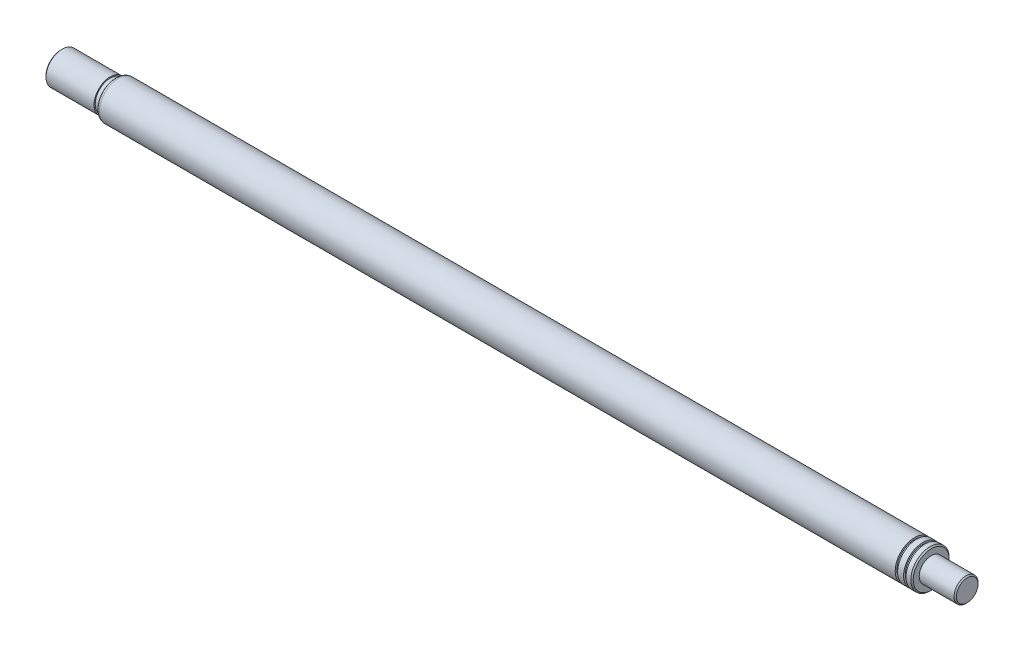
from build123d import *


with BuildPart() as part:
    # 草图1 → 旋转1 (revolve)
    with BuildSketch(Plane.XY, mode=Mode.PRIVATE) as revolve_1_sk:
        with BuildLine():
            Line((0, 0), (0, 12.5))
            Line((0, 12.5), (1, 13.5))
            Line((1, 13.5), (41, 13.5))
            Line((41, 13.5), (41, 12.5))
            Line((41, 12.5), (45, 12.5))
            Line((45, 12.5), (45, 13))
            ThreePointArc((45, 13), (45.878679656, 15.121320344), (48, 16))
            Line((48, 16), (711, 16))
            Line((711, 16), (711, 14.5))
            Line((711, 14.5), (713, 14.5))
            Line((713, 14.5), (713, 16))
            Line((713, 16), (718, 16))
            Line((718, 16), (718, 14.5))
            Line((718, 14.5), (720, 14.5))
            Line((720, 14.5), (720, 16))
            Line((720, 16), (724, 16))
            Line((724, 16), (725, 15))
            Line((725, 15), (725, 10))
            Line((725, 10), (754, 10))
            Line((754, 10), (755, 9))
            Line((755, 9), (755, 0))
            Line((755, 0), (0, 0))
        make_face()
    revolve(revolve_1_sk.sketch.rotate(Axis((0, 0, 0), (1, 0, 0)), 90), axis=Axis((0, 0, 0), (1, 0, 0)))


solid = part.part
